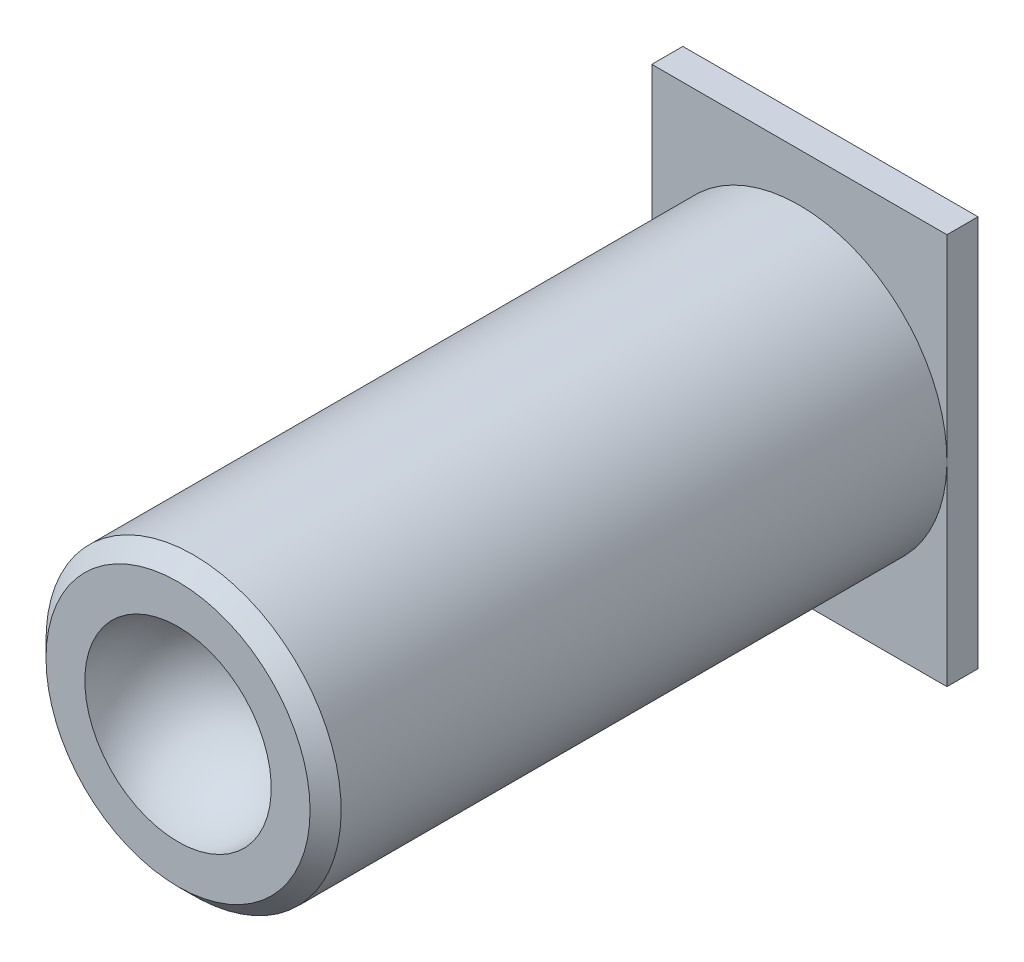
from build123d import *

# Parameters (mm, degrees)
SKETCH1_W           = 95
SKETCH1_H           = 126
BOSS_EXTRUDE1_DEPTH = 10


with BuildPart() as part:
    # Sketch1 → Boss-Extrude1 (new body)
    with BuildSketch(Plane.XY):
        Rectangle(SKETCH1_W, SKETCH1_H)
    extrude(amount=BOSS_EXTRUDE1_DEPTH)


with BuildPart() as body_2:
    # Sketch3 → Revolve1 (revolve)
    with BuildSketch(Plane(origin=(0, 0, 0), x_dir=(0, 0, -1), z_dir=(1, 0, 0))):
        with BuildLine():
            Line((-10, 0), (-10, 47.5))
            Line((-10, 47.5), (-205, 47.5))
            Line((-205, 47.5), (-210, 42.5))
            Line((-210, 42.5), (-210, 30))
            ThreePointArc((-210, 30), (-188.786796564, 21.213203436), (-180, 0))
            Line((-180, 0), (-10, 0))
        make_face()
    revolve(axis=Axis((0, 0, 10), (0, 0, 1)))


solid = Compound([part.part, body_2.part])
